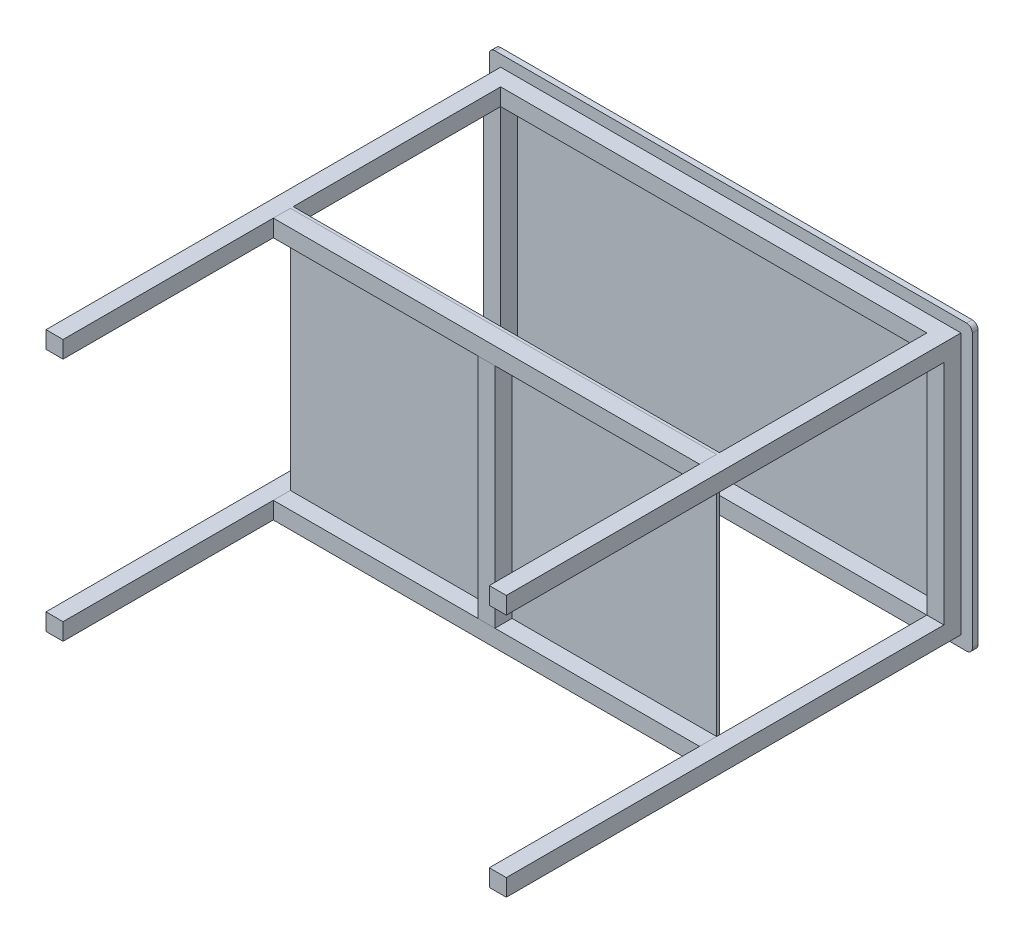
from build123d import *

# Parameters (mm, degrees)
SKETCH_1_W      = 850
SKETCH_1_H      = 500
EXTRUDE_1_DEPTH = 10
SKETCH_2_W      = 810
SKETCH_2_H      = 460
SKETCH_2_W_2    = 750
SKETCH_2_H_2    = 400
EXTRUDE_2_DEPTH = 30
SKETCH_3_W      = 30
SKETCH_3_H      = 30
EXTRUDE_3_DEPTH = 770
EXTRUDE_START   = -460
SKETCH_4_W      = 750
SKETCH_4_H      = 5
EXTRUDE_4_DEPTH = 460
SKETCH_6_W      = 750
SKETCH_6_H      = 30
EXTRUDE_7_DEPTH = 30
SKETCH_7_W      = 750
SKETCH_7_H      = 30
EXTRUDE_8_DEPTH = 30
SKETCH_8_W      = 30
SKETCH_8_H      = 400
EXTRUDE_9_DEPTH = 30
FILLET_1_R      = 10


with BuildPart() as part:
    # 草图1 → 凸台-拉伸1 (new body)
    with BuildSketch(Plane.XY):
        Rectangle(SKETCH_1_W, SKETCH_1_H)
    extrude(amount=EXTRUDE_1_DEPTH)

    # 圆角1
    fillet_1_edges = [part.edges().sort_by_distance(p)[0] for p in [
        (425, -250, 5),
        (-425, -250, 5),
        (-425, 250, 5),
        (425, 250, 5),
    ]]
    fillet(fillet_1_edges, radius=FILLET_1_R)


with BuildPart() as body_2:
    # 草图2 → 凸台-拉伸2 (new body)
    with BuildSketch(Plane.XY.offset(10)):
        Rectangle(SKETCH_2_W, SKETCH_2_H)
        Rectangle(SKETCH_2_W_2, SKETCH_2_H_2, mode=Mode.SUBTRACT)
    extrude(amount=EXTRUDE_2_DEPTH)

    # 草图3 → 凸台-拉伸3 (add)
    with BuildSketch(Plane.XY.offset(40)):
        with Locations((-390, 215)):
            Rectangle(SKETCH_3_W, SKETCH_3_H)
        with Locations((390, -215)):
            Rectangle(SKETCH_3_W, SKETCH_3_H)
        with Locations((390, 215)):
            Rectangle(SKETCH_3_W, SKETCH_3_H)
        with Locations((-390, -215)):
            Rectangle(SKETCH_3_W, SKETCH_3_H)
    extrude(amount=EXTRUDE_3_DEPTH)

    # 草图4 → 凸台-拉伸4 (add)
    with BuildSketch(Plane(origin=(0, 230, 0), x_dir=(1, 0, 0), z_dir=(0, 1, 0)).offset(EXTRUDE_START)):
        with Locations((0, -407.5)):
            Rectangle(SKETCH_4_W, SKETCH_4_H)
    extrude(amount=EXTRUDE_4_DEPTH)


with BuildPart() as body_3:
    # 草图6 → 凸台-拉伸7 (new body)
    with BuildSketch(Plane.XZ.offset(230)):
        with Locations((0, 425)):
            Rectangle(SKETCH_6_W, SKETCH_6_H)
    extrude(amount=-EXTRUDE_7_DEPTH)


with BuildPart() as body_4:
    # 草图7 → 凸台-拉伸8 (new body)
    with BuildSketch(Plane(origin=(0, 230, 0), x_dir=(1, 0, 0), z_dir=(0, 1, 0))):
        with Locations((0, -425)):
            Rectangle(SKETCH_7_W, SKETCH_7_H)
    extrude(amount=-EXTRUDE_8_DEPTH)


with BuildPart() as body_5:
    # 草图8 → 凸台-拉伸9 (new body)
    with BuildSketch(Plane.XY.offset(440)):
        Rectangle(SKETCH_8_W, SKETCH_8_H)
    extrude(amount=-EXTRUDE_9_DEPTH)


solid = Compound([part.part, body_2.part, body_3.part, body_4.part, body_5.part])
